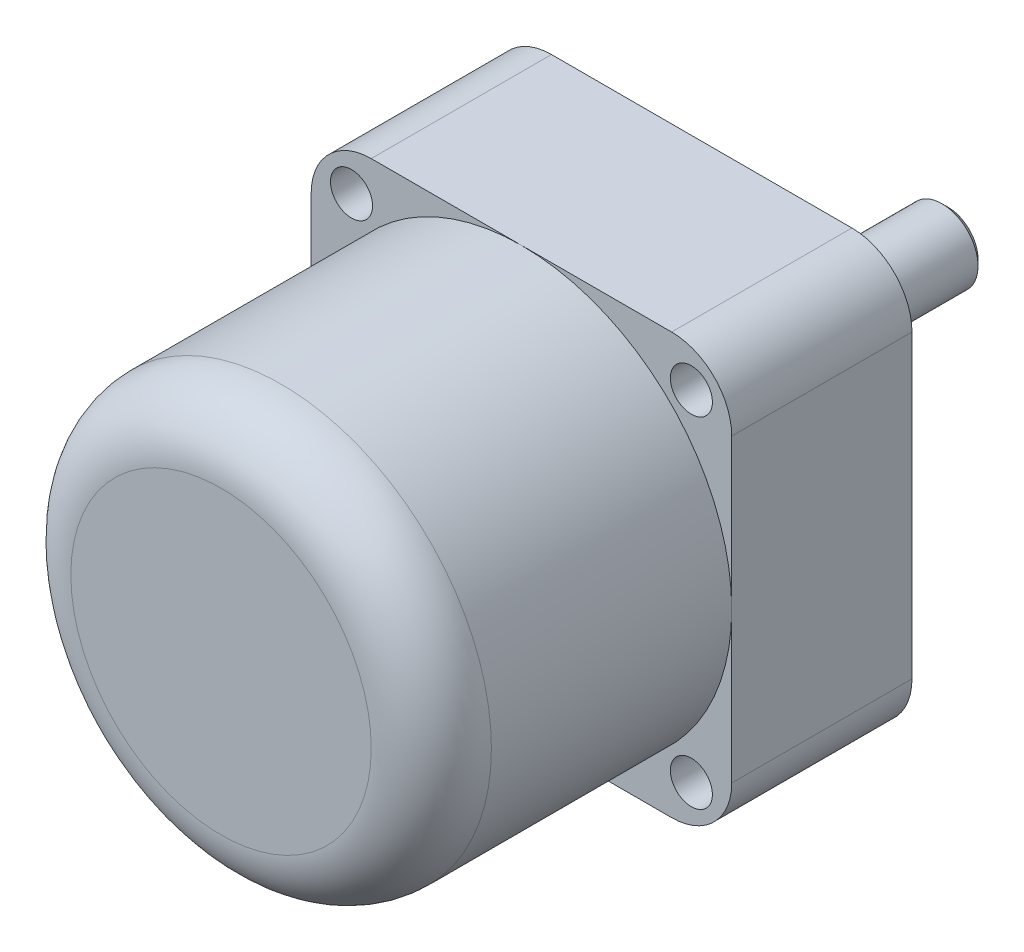
SolidWorks part; units mm, degrees
ref_plane "Front Plane" through (0, 0, 0) normal (0, 0, 1) x (1, 0, 0)
ref_plane "Top Plane" through (0, 0, 0) normal (0, 1, 0) x (1, 0, 0)
ref_plane "Right Plane" through (0, 0, 0) normal (1, 0, 0) x (0, 0, -1)
sketch "Sketch1" plane through (0, 0, 0) normal (0, 0, 1) x (1, 0, 0)
  line L1 (35, -35) -> (-35, -35)
  line L2 (35, -35) -> (35, 35)
  line L3 (35, 35) -> (-35, 35)
  line L4 (-35, -35) -> (-35, 35)
  line L5 (35, -35) -> (-35, 35) construction
  line L6 (35, 35) -> (-35, -35) construction
  point P1 (0, 0)
  dimension "D1" = 70
  dimension "D2" = 70
extrude "Boss-Extrude1" add sketch "Sketch1" along normal blind 30
sketch "Sketch2" plane through (0, 0, 30) normal (0, 0, 1) x (1, 0, 0)
  circle A0 centre (0, 0) radius 27.5
  dimension "D1" = 55
fillet "Fillet2" radius 10 4 edges at (35, -35, 15) (-35, -35, 15) (35, 35, 15) (-35, 35, 15)
sketch "Sketch3" plane through (0, 0, 30) normal (0, 0, 1) x (1, 0, 0)
  line L0 (0, 0) -> (-32.0711, 32.0711) construction
  arc A1 (-25, 35) -> (-35, 25) centre (-25, 25) ccw construction
  circle A2 centre (-28.2843, 28.2843) radius 3.5
  dimension "D2" = 7
extrude "Cut-Extrude1" cut sketch "Sketch3" against normal blind 60
sketch "Sketch4" plane through (0, 0, 0) normal (0, 0, -1) x (-1, 0, 0)
  circle A0 centre (0, 0) radius 22.5
  dimension "D1" = 45
extrude "Boss-Extrude3" add sketch "Sketch4" along normal blind 6
sketch "Sketch5" plane through (0, 0, -6) normal (0, 0, -1) x (-1, 0, 0)
  circle A0 centre (0, 0) radius 6
  dimension "D1" = 12
extrude "Boss-Extrude4" add sketch "Sketch5" along normal blind 35
chamfer "Chamfer1" distance 1 angle 45 1 edges at (-6, 0, -41)
chamfer "Chamfer2" distance 1 angle 45 1 edges at (-22.5, 0, -6)
pattern_circular "CirPattern1" count 4 over 360 about axis through (0, 0, 0) along (0, 0, 1) of "Cut-Extrude1"
sketch "Sketch6" plane through (0, 0, 30) normal (0, 0, 1) x (1, 0, 0)
  circle A0 centre (0, 0) radius 35
  dimension "D1" = 70
extrude "Boss-Extrude5" add sketch "Sketch6" along normal blind 50
fillet "Fillet3" radius 10 1 edges at (35, 0, 80)
